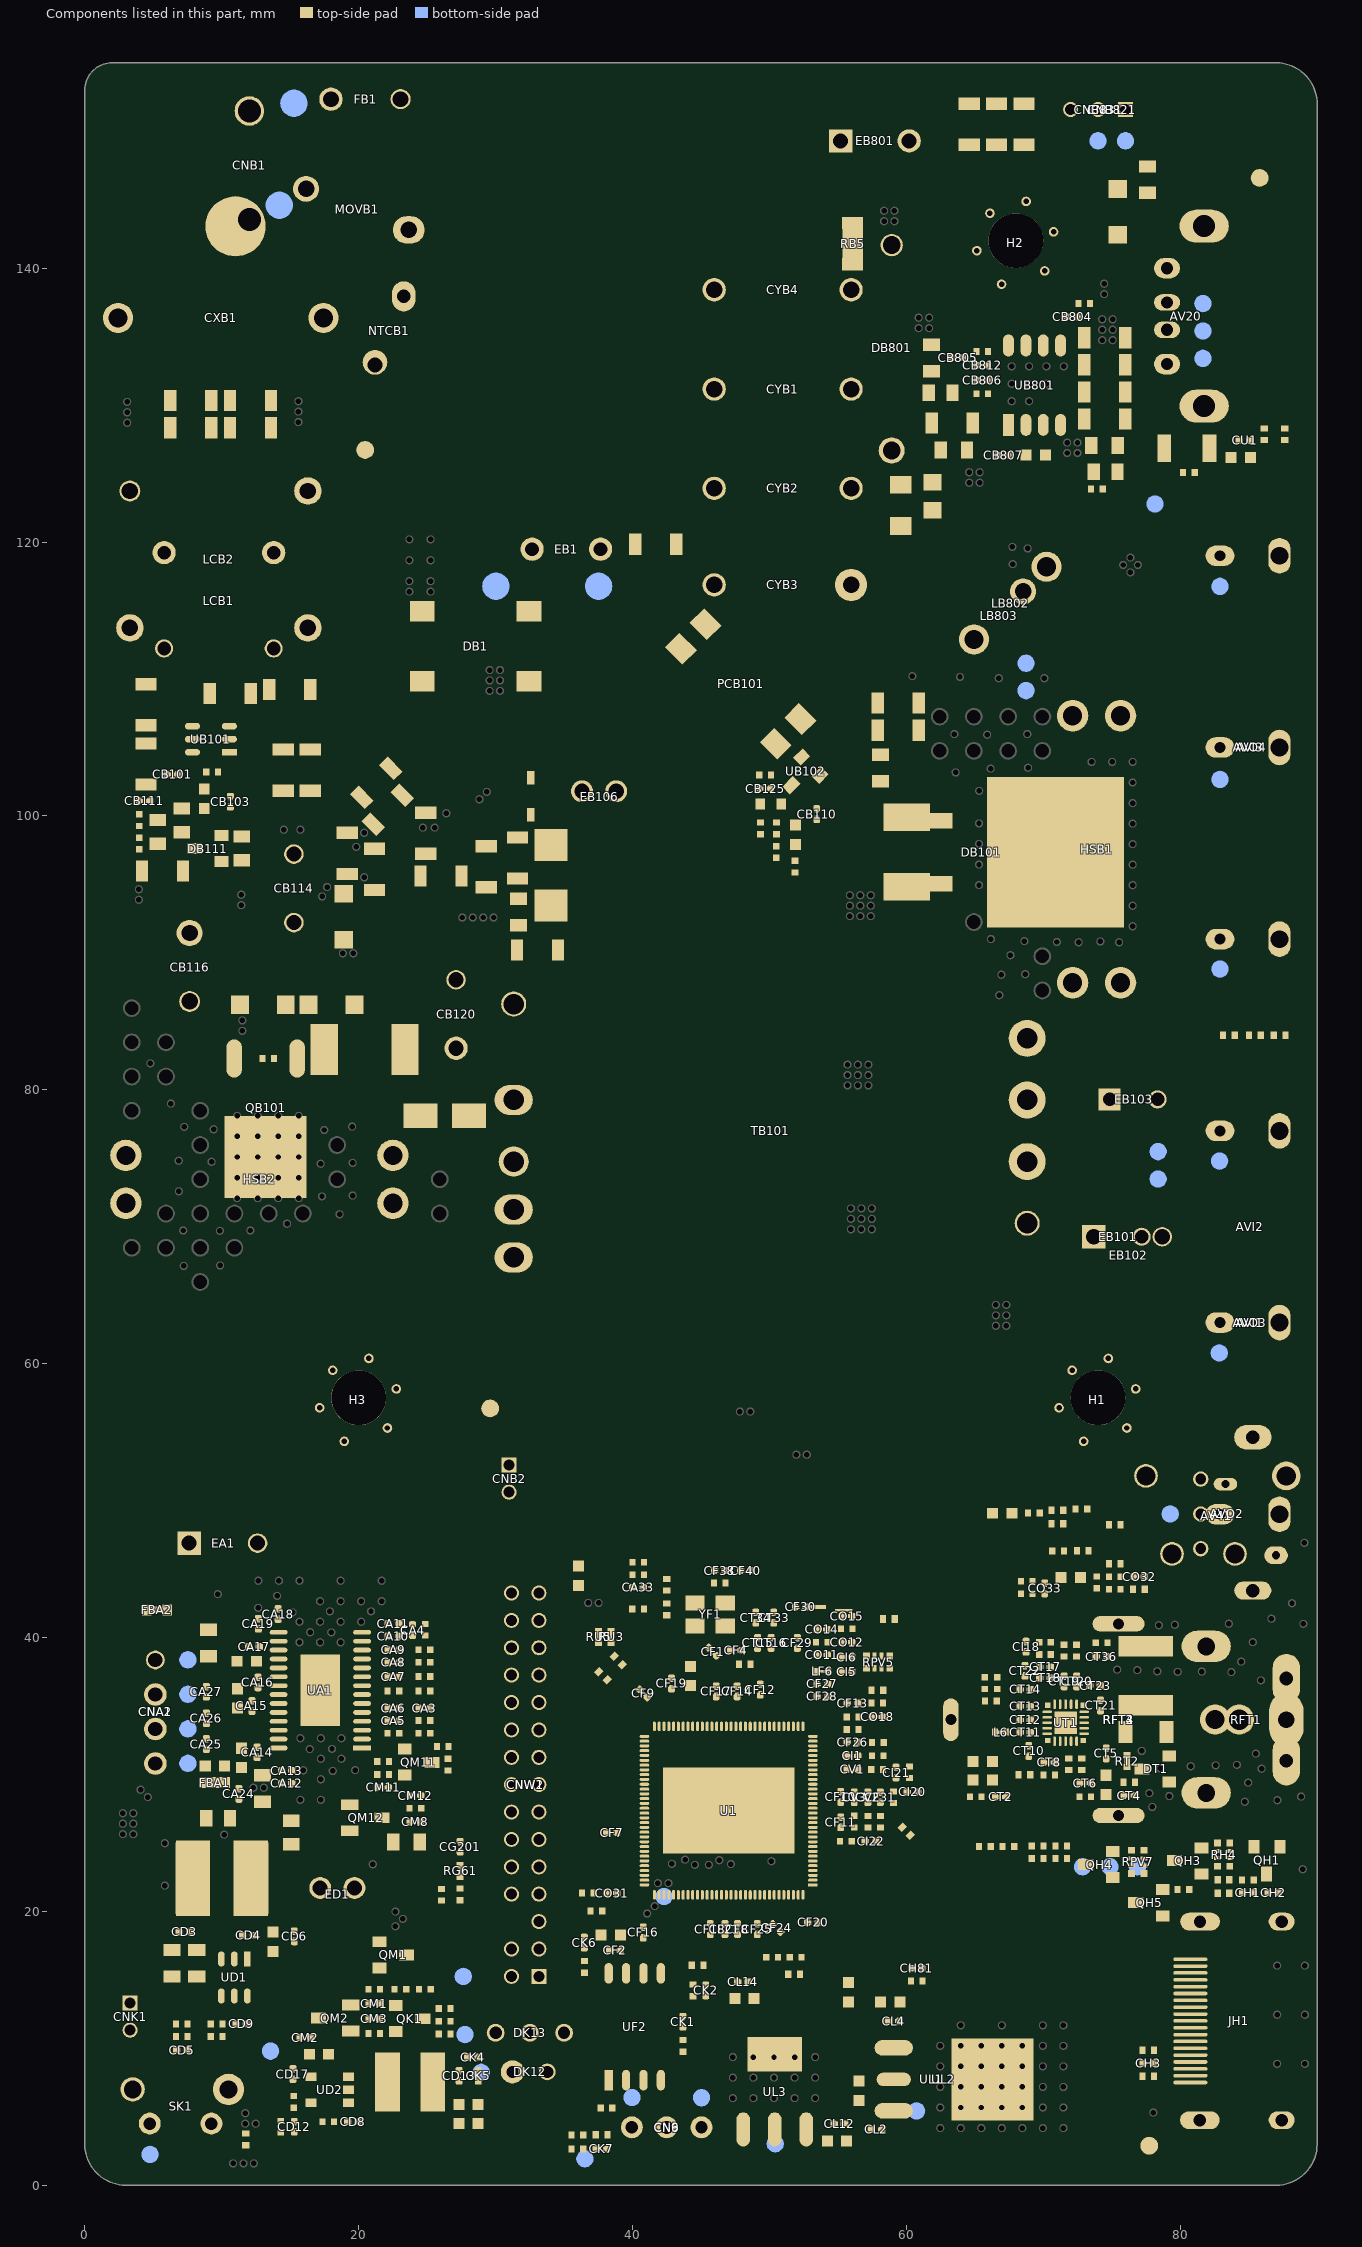
[diagram p0: the components of this part, seen from the top]
# Altium PCB MISC116569.PcbDoc (part 5 of 15)
Units mm, origin at the board's own origin, x right, y up, seen from the top; angles counter-clockwise.
Board outline 90 x 155 mm, 2 copper layers (TopLayer, BottomLayer), stack 1.571 mm thick; 527 components, 277 nets, 2450 pads, 649 vias.

## Footprints (in the part's own frame and the unit in brackets; to place one, negate y for a bottom-side part, rotate by r counter-clockwise, add the part's x,y. Pads: shape width x height; smd on the part's side, far side on the other; paste and mask are expansions set on the pad) (continued)
TO-252 [mm] "与TO-223兼容；15.12.29"
  oval 1.143x2.794 smd: 1(-2.3,-3.6) 3(2.3,-3.6)
  rect 6x6 smd paste-10: 2(0,3.6)
  rect 4x2.6 on Top Paste: 4(0,1.957)
  TopLayer pour cut-out: 2.3,-1.932 2.3,-5.055 -2.345,-5.055 -2.64,-4.996 -2.891,-4.829 -3.058,-4.579 -3.117,-4.284 -3.117,-4.284 -2.299,-4.284 -2.299,-2.699 -3.124,-2.699 -3.066,-2.406 -2.899,-2.157 -2.65,-1.99 -2.356,-1.932 -2.356,-1.932
  silkscreen extent -3.4,-1.34 3.4,7.01, body extent -3.4,-4.15 3.4,6.05, height 2.5
TO-252-GDS [mm] "SC08440  IRLR024N"
  rect 6x6 smd: D(0,0)
  oval 1.143x2.794 smd: G(-2.3,-7.2) S(2.3,-7.2)
  silkscreen extent -3.4,-5.64 3.4,3.4, body extent -3.4,-7.75 3.4,2.45, height 2.5
TP [mm] "TEST POINT   (不带paste  1.27mm 直径）"
  round 1.27 smd paste-1.27: 1(0,0)
TP-80 [mm] "TEST POINT;2mm"
  round 2 smd paste-1.27: 1(0,0)
TP-TDT [mm] "电源放电测试点，间隔7.5mm"
  round 2 smd paste-2: 1(-3.75,0) 2(3.75,0)
  silkscreen extent -5.75,-2 5.75,2
TP_BL [mm] "TEST POINT,专用背光测试点"
  round 1.27 smd paste-1.27: 1(0,0)
  silkscreen extent -6.4,-0.97 0.95,0.96
TSOT23-6 [mm] "MP65151DJ[MPS]/MP1470"
  rect 1.1x0.5 smd: 1(-1.35,0.95)
  oval 1.1x0.5 smd: 2(-1.35,0) 3(-1.35,-0.95) 4(1.35,-0.95) 5(1.35,0) 6(1.35,0.95)
  silkscreen extent -1.08,-1.5 0.85,2.8, body extent -0.85,-1.5 0.85,1.5, height 1
USB1-HD-2 [mm] "捷仕泰 ： U2504M-04-E1WD-C；170204加宽后壳丝印(18.03.12,更新信号脚孔径）"
  oval 2.7x3.9 on Top Overlay: 0(-6.57,10.257) 0(6.57,10.247)
  oval 1.7x2.1 on Top Overlay: 0(-3.5,12.957) 0(3.5,12.957)
  oval 1.5x1.9 hole 0.9 slot 1.4 at 90 deg: 1(-3.5,12.957) 4(3.5,12.957)
  oval 1.4x2.1 on Top Overlay: 1(-1,12.957) 2(1,12.957)
  oval 1.2x1.9 hole 0.9 slot 1.4 at 90 deg: 2(-1,12.957) 3(1,12.957)
  oval 2.4x3.6 / inner oval 2.4x3.6 / far side oval 2.8x4 hole 1.6 slot 2.3 at 90 deg: 5(6.57,10.247) 6(-6.57,10.247)
  TopLayer pour cut-out: 2.433,14.667 4.428,14.667 4.532,14.647 4.62,14.588 4.678,14.5 4.699,14.396 4.699,14.396 4.699,11.335 4.68,11.238 4.625,11.156 4.542,11.101 4.445,11.081 4.445,11.081 2.422,11.081 2.422,14.656
  KeepOutLayer pour cut-out: -3.49,14.696 -4.146,14.566 -4.703,14.194 -5.075,13.637 -5.206,12.98 -5.206,12.98 -5.206,12.94 -5.068,12.25 -4.677,11.665 -4.092,11.275 -3.402,11.137 -3.402,11.137 2.42,11.137 2.637,11.18 2.821,11.303 2.943,11.487 2.986,11.703 2.986,11.703 2.986,14.149 2.944,14.361 2.824,14.541 2.644,14.661 2.432,14.704 2.432,14.704 -3.482,14.704 -3.485,14.703 -3.487,14.701 -3.489,14.699 -3.49,14.696
  silkscreen extent -7.1,2.04 7.05,14.58, body extent -10,-87.25 10,14.14, height 8.2
VR(13*5)-V-7.5 [mm] "为勤,VARISTOR,17.01.04修改为椭圆孔;160105更新椭圆孔 //0424_2019在顶层加整块白油,"
  oval 2.311x2 / inner oval 2.8x2 / far side oval 2.8x2 hole 1.2 slot 2 at 0 deg: 1(3.75,-1.5)
  round 1.9 hole 1.2: 2(-3.75,1.5)
  round 2.1 on Top Overlay: 2(-3.75,1.5)
  oval 3x2.2 on Top Overlay: 2(3.75,-1.5)
  silkscreen extent -6.65,-2.5 6.44,2.5, body extent -6.5,-2.75 6.5,2.75, height 15.5
XTAL-S-3 [mm] "三星（SQ3D03200D2IBA）晶振"
  rect 1.4x1.1 smd: 1(-1.1,-0.85) 2(1.1,-0.85) 3(1.1,0.85) 4(-1.1,0.85)
  silkscreen extent -2.37,-1.91 1.65,1.3, body extent -1.65,-1.3 1.65,1.3, height 0.8

## Part data
5V CVBS_IN DM0 DP0 GND LOUT+ LOUT- PWM_REF ROUT+ ROUT- TP_12VA+ TP_12VA- TP_12VB+ TP_12VB- TP_L TP_LED+ TP_LED- TP_N UART_RX UART_TX Y_Pb_LOUT Y_Pr_ROUT Y_Y_AV_OUT YPBPR_L/AV_L YPBPR_R/AV_R: library part TEST
AV20: library part XXX.XXX.0002687, "USB jack,USB Jack,H,Single,flange,DIP,103411271,VAST-DLMI"
AV41: library part XXX.XXX.0002138, "Earphone jack,Earphone Jack,H,Φ3.5,CH7.0,Black,switch,Seal,DIP,PJ7724-F05L3BY-D,YUQIU-DLMI"
AVI1 AVO4: library part "RCA端子,RCA Jack,AV3,H,Yellow、White、Red,CH5.5,D14,Seal,DIP,RC075-F03L3BY-A,YUQIU-DLMI-AV", "CN-AV-D14-#-#"
AVI2: library part "RCA端子,RCA Jack,AV2,H,White、Red,CH5.5,D14,Seal,DIP,AV63-02S-0030,QS(MI手插物料)-DLMI-AUDIO", "CN-AUDIO-D14-#-#"
AVI3: library part "RCA端子,RCA Jack,AV3,H,Green、Blue、Red,CH5.5,D14,Seal,DIP,RC075-F03L3BY-B,YUQIU-DLMI-YPbPr", "CN-YPbPr-D14-#-#"
AVO2: library part GQ-03-08-DLMI, "CN-DLMI-optical fiber"
AVO3: library part "RCA端子,RCA Jack,AV3,H,Orange、White、Red,CH5.5,D14,Seal,DIP,RC075-F03L3BY-C,YUQIU-DLMI"
BA1 BA2 BA3 BA4: library part 004.004.0000104-D, "Multilayer inductor,HF Inductor,220nH,±5%,0603,SMD,SWI0603F-R22J,Tai-tech-D"
BB101: library part 004.004.0001046-D, "Ferrite bead,BEAD,50ohm,3.0×4.0,9A,SMD,TP,SMB-302540-K5B-L1,SOLDIER-D"
BB801: library part UPZ2012E601-2R0TF(600ohm-2000mA)
BB802: library part 004.004.0000340-D, "Ferrite bead,BEAD,600ohm±25%,0805,2000mA,SMD,TP,UPZ2012E601-2R0TF,Sunlord-D"
BOE: library part PCB_NAME
CA1 CA2 CD1 CD2 CM7: library part 004.003.0000386-D, "Ceramic capacitor,CAP MC,16V,10uF,±20%,X5R,0805,SMD,TP-D"
CA3 CA4: library part 004.003.0000549-D, "Ceramic capacitor,CAP MC,50V,3300pF,±10%,X7R,0402,SMD,TP-D"
CA5 CA6 CA10 CA11 CA14 CA15 CA16 CA17: library part 004.003.0000398-D, "Ceramic capacitor,CAP MC,16V,0.22uF,±20%,X5R,0402,SMD,TP-D"
CA7 CA9: library part 004.003.0000402-D, "Ceramic capacitor,CAP MC,16V,1uF,±20%,X5R,0402,SMD,TP-D"
CA8 CA12 CA18 CD3 CD4 CD6 CD8 CD9 CL2 CL12 CM1 CM2 CM8 CO32: library part 004.003.0000403-D, "Ceramic capacitor,CAP MC,16V,0.1uF,±20%,X5R,0402,SMD,TP-D"
CA13 CA19: library part 004.003.0000503-D, "Ceramic capacitor,CAP MC,50V,1000pF,±10%,X7R,0402,SMD,TP-D"
CA24 CA25 CA26 CA27: library part 004.003.0000534-D, "Ceramic capacitor,CAP MC,50V,2200pF,±10%,X7R,0402,SMD,TP-D"
CA31 CA32 CD7 CL13: library part 004.003.0000383-D, "Ceramic capacitor,CAP MC,6.3V,10uF,±20%,X5R,0603,SMD,TP-D"
CA33 CO12 CO15: library part 004.003.0000361-D, "Ceramic capacitor,CAP MC,6.3V,0.47uF,±10%,X5R,0402,SMD,TP-D"
CB101 CB111 CB807: library part 100pF-0402-NPO-±5%-50V-D
CB102 CB109: library part 0.1uF-0603-X7R-±10%-50V-D, "CAP"
CB103 CB806 CF29 CF30 CO11 CO14 CO18: library part 1000pF-0402-X7R-±10%-50V-D
CB110 CB125: library part 1000pF-0402-X7R-±10%-50V-D, "CAP"
CB113 CB808 CB809 CB810 CB811: library part 220PF-0805-NPO-±10%-200V-D, "CAP"
CB114: library part C242G472J20A201(编带/法拉)-DAI, "CAP"
CB116: library part 004.003.0001889-DHAI, "Ceramic capacitor,CAP CD,1KV,100pF,±5%,SL,OK,5.0mm,DIP,TP,TDK-DHAI"
CB118: library part 1000pF-0805-NPO-±10%-200V-D, "CAP"
CB120: library part 004.003.0001665, "Ceramic capacitor,CAP CD,1KV,4700pF,±20%,Y5U,K,5.0mm,DIP,TP,Walsin-DHAI"
CB801: library part 1uf-0603-X7R-±10%-25V-D
CB804: library part 4700pF-0402-X7R-±10%-50V-D
CB805: library part 0.1uF-0402-X7R-±10%-16V-D
CB812: library part 0.033uF-0402-X7R-±10%-16V-D
CD5: library part 004.003.0000570-D, "Ceramic capacitor,CAP MC,50V,56pF,±5%,NPO,0402,SMD,TP-D"
CD10 CD14 CD15 CD16 CF3 CF5 CF15 CL1 CL3 CL11 CT1 CT52 CU2: library part 10uF-0603-X5R-±20%-6.3V-D
CD12: library part 3300pF-0402-X7R-±10%-50V-D
CD13 CD17 CH1 CH2 CK4 CK5 CM11: library part 0.1uF-0402-X5R-±20%-16V-D
CF1 CF4: library part 004.003.0000527-D, "Ceramic capacitor,CAP MC,50V,18pF,±5%,NPO,0402,SMD,TP-D"
CF2 CF7 CF8 CF9 CF10 CF12 CF13 CF14 CF17 CF27 CG201 CI5 CI6 CK1 CT2 CT4 CT5 CT6 CT7 CT8 CT9 CT10 CT11 CT12 CT15 CT16 CT17 CT18 CT21 CT22 CT23: library part 0.1uF-0402-Y5V-+80%-20%-16V-D
CF11 CF16 CF18 CF19 CF20 CF21 CF25 CF28 CH81 CK7 CU1: library part 1uF-0402-X5R-±20%-6.3V-D
CF24: library part 004.003.0000100-D, "Ceramic capacitor,CAP MC,6.3V,2.2uF,±20%,X5R,0402,SMD,TP-D"
CF26 CF31 CI1 CV1 CV2 CV3: library part 0.047uF-0402-X7R-±10%-16V-D
CF38 CF40 CI18: library part 30pF-0402-NPO-±5%-50V-D
CH3: library part 004.003.0000530-D, "Ceramic capacitor,CAP MC,50V,22pF,±5%,NPO,0402,SMD,TP-D"
CI20 CI21 CI22 CK6: library part 10pF-0402-NPO-±5%-50V-D
CK2: library part 0.01uF-0402-X7R-±10%-50V-D
CL4 CL14: library part 004.003.0000382-D, "Ceramic capacitor,CAP MC,6.3V,1uF,±20%,X5R,0402,SMD,TP-D"
CM3 CM12: library part 0.022uF-0402-X7R-±10%-16V-D
CN6: library part 004.008.0000361-DHMI, "IR receiver,IR Receriver,2.5V~6V,38K,DIP,FDI-M6069560R538-WJGC25-D22,Fantasy-DHMI"
CN9: library part 004.008.0000501-DHMI, "IR receiver,IR Receriver,DIP,ARM-383AW1-Z-R-D10-22,ALL-BEST-DHMI"
CNA1: library part XXX.XXX.0000595-DHMI, "Connector socket,connect jack,4Pin,D2.50,D,L=2.8mm,DIP,CNJST-DHMI"
CNA2: library part XXX.XXX.0000676-DHMI, "Connector socket,connect jack,4Pin,D2.54,D,SNAP,L=3.0mm,DIP,BOOM-DHMI"
CNB1: library part "连接插座,connect jack,2Pin,D7.92,L,SNAP,Fool-proofing,nature,L=2.8mm,DIP,AMA-DLMI", "AC socket"
CNB2: library part XXX.XXX.0001753, "Connector socket,connect jack,2Pin,D2.0,D,L=2.8mm,DIP,AMA-DHMI"
CNB821: library part XXX.XXX.0000603-DHMI, "Connector socket,connect jack,2Pin,D2.0,D,L=3.4mm,DIP,BOOM-DHMI"
CNB831: library part XXX.XXX.0000643-DHMI, "Connector socket,connect jack,3Pin,D2.0,D,SNAP,L=2.8mm,DIP,CNJST-DHMI"
CNK1: library part 2PIN-2.0-D-H-G-B-DHMI, "Socket"
CNW1: library part 2×15PIN-2.0-D-H-M(脚长=2.6mm)(缺6PIN)-LK-DHMI, "CN-straight pin header"
CNW2: library part "连接插座,connect jack,2×15Pin/without pin6,D2.0,D,SNAP,Fool-proofing,Nature,L=2.6mm,DIP,CJ", "CN-with latch"
CO31 CT13 CT14 CT19 CT20 CT33 CT34 CT36: library part 33pF-0402-NPO-±5%-50V-D
CO33: library part 330pF-0402-NPO-±5%-50V-D
"Conformal Coating": library part 三防漆,25kg/Can,Peters
CT3: library part 1000pF-1206-X7R-±20%-2000V-D
CXB1: library part "X电容,CAP X2,MP,275VAC,0.47uF,±10%,S,15mm-Mini,PC,DIP,BM-DHMI", "CAP"
CYB1 CYB2 CYB3 CYB4: library part "Y电容,CAP Y1,CD,470pF,400VAC,±20%,KS,10mm,Y5U,DIP,Walsin-DHMI", "Y1 capacitor"
D101 D102 DA31 DA32 DA33 DI10 DI11 DK1 DK3 DV3 DV4 DV5 DV7 DV8 DV9: library part AVLC18S02003-D
DAS1: library part DOLBY_AS2
DB1: library part 004.005.0000860-D, "Bridge rectifier,DIO BRD,3A,800V,YBS,SMD,YBS3010A,YJ-D"
DB101: library part MBRB10150CT(GOOD-ARK)-D, "Diode"
DB104: library part M7(GOOD-ARK)-D
DB106 DB109 DB110 DB804: library part "整流二极管,DIO FRD S,1.2A,800V,eSGA,SMD,R12K,GOOD-ARK-D"
DB111: library part LBAV70LT1G(LRC)-D, "Diode"
DB121: library part BAV21WS-D, "Diode"
DB801: library part SR210(编带/台半)-DLAI, "Diode"
DH1 DH2 DH3 DH81: library part 004.005.0000315-D, "TVS diode,DIO ESD,2.5pF,200V,0402,SMD,SFI0402-240E-2R5PP-LF,SFI-D"
DI1 DI2 DI3: library part AIES12U020R2-D
DK12: library part "发光二极管,Single LED,RED,25mA,28mcd,638nm,1.9V,φ3.85×5.4mm,DIP,HL-DLMI"
DK13: library part WEJ3290C-R3H8-BC(红、绿)-高亮-DLMI
DT1: library part BAV99-BR-D
DU1 DU2 DU3 DU4: library part 004.005.0000203-D, "TVS diode,DIO ESD,0.2pF,25V,0402,SMD,AIES12U020R2,AMOTECH-D"
EA1: library part 004.003.0000601-DHAI, "Aluminum electrolytic capacitor,CAP AL,16V,470uF,±20%,RK,P,5.0mm,10×12,DIP,TP,XL-DHAI"
EB1: library part 47uF-400V-±20%-13×30-105℃-KY-折脚(H=11mm)(Capxon)-DLMI, "Electrolytic"
EB101 EB103: library part 270uF-16V-±20%-8×11.5-105℃-PS-短脚-F=3.5(Capxon), "Solid-state"
EB102: library part 470uF-25V-±20%-10×12.5-105℃-GF-编带-F=5.0(CapXon)-DHAI, "Electrolytic"
EB106: library part 10uF-50V-±20%-5×11-105℃-GH-编带-F=2.5(CapXon)-DHAI, "Electrolytic"
EB801: library part 47uF-100V-±20%-10×12-105℃-EV-编带-F=5.0(Elite)-DHAI, "Electrolytic"
ED1: library part 470uF-10V-±20%-6.3×11-105℃-黑底白字-编带-F=2.5-XF-DHAI, "Electrolytic"
EVA1 EVA2 EVA3 EVA4: library part 7×7×3mm-C-4305防火泡棉-黑色-DLMI, "EVA"
FB1: library part 004.026.0000010-DHMI, "Slow-blow fuse,FUSE T,P,3.15A,250VAC,8.5×4.0×8mm,DIP,TP,Walter-DHMI"
FBA1 FBA2: library part 0ohm-0603-PCB-D, "0ohm-0603-PCB-D"
FT2 LT1 LT3 LT4: library part SDCL1005CR27JTDF(顺络)-D
FU1: library part 004.026.0000039-D, "Resettable fuse,FUSE PTC,1.1A,6V,1206,SMD,TP,TLC-D"
GD1 GD2 GD3: library part 7.00×8.35mm-尼龙-白色-WQM-DHMI, "Mylar stud"
GDT1: library part 004.005.0000675, "Gas discharge tube,GDT,700V,2000A,TP,4.5*3.2mm,SMD,4532-091-LF,Brightking-D"
GL1 GL5 GL6 GL7 GL8: library part 005.002.0000011, "Silicone,0.2g,general purpose,60,White,SLD-8854W,XY-DHMI"
GL3 GL4: library part 005.002.0000011-D-5*3mm, "Silicone,0.5g,general purpose,60,White,SLD-8854W,XY-D"
H1 H2 H3: library part "Location hole-D"
HS1: library part 004.040.0008928-D, "Heat sink,15.0×15.0×5.0mm,AL1060H-24,Black,high-emissivity paint spray,stamped with bends,no rivet pins,YT-D"
HSB1 HSB2: library part 004.040.0006600-DHMI, "Heat sink,17.5×14.5×0.5mm,copper sheet,matte tin plated,natural color,four pins,WT-DHMI"
JH1: library part XXX.XXX.0001122-D, "HDMI jack,HDMI Jack,H,SMD,161031041(hull-SPCC ),VAST-D"
L3: library part FCM1005KF-121T06(120ohm-500mA)-D
L6 LF6 RG61 RT2 RU3 RU5: library part 0ohm-0402-PCB-D, "0ohm-0402-PCB-D"
LB802: library part SYDR1212-L003-HM-DHMI, "I-core inductor"
LB803: library part 差模电感,Inductor,DR12×14,68uH,0.45,20Ts,H13.5MAX,SYDR1214-L068uA,DIP,Soldier-DHMI, "I-core inductor"
LCB1: library part SYUU9.8-L002-JM-DLMI, "Common mode"
LCB2: library part SYUU10.5-L002-JM-DHMI, "Common mode"
LD1: library part 004.004.0000017-D, "Power inductor,Power Inductor,4.7uH,±20%,2.8A,0.35×1P,DR5.8×4.5,SMD,SCD54TL-4R7M,Soldier-D"
LD2: library part SLN43T-6R8M-D
LD3: library part 004.004.0000016-D, "Power inductor,Power Inductor,4.7uH,±20%,3.3A,DR6.0×4.5,SMD,SWPA6045S4R7MT,Sunlord-D"
LT2: library part MGLB1608M121T2R0-LF(120ohm-2000mA)-D
M1 M2 M3 M4: library part MARK-D
ML1: library part MALAY
MOVB1: library part TVR10561KSW(为勤)-DHMI, "Varistor"
NTCB1: library part SCK102R55AMBY502(短脚/为勤)-DHMI, "Thermistor"
PCB101: library part LTV-817S-TA-B(光宝)-DMI, "Optocoupler"
QB101: library part 场效应管,NMOS,5.2,650V,1.02ohm@ID=2.6A@VGS=10V,DPAK,TK5P65W,TOSHIBA-D, "N Channel Single MOSFET"
QH1 QM1: library part 004.006.0000007-D, "General-purpose transistor,Dynatron,NPN,0.2A,40V,60-300,SOT-23,KMBT3904,KEXIN-D"
QH3 QH4 QH5 QK1 QM11: library part LMBT3904LT1G-D-NPN, "Q-NPN-#-#-#"
QM2: library part 004.007.0000286-D, "MOSFET,PMOS,-4.7A,-20V,70mohm@ID=-4.7A@VGS=-4.5V,SOT23-LC,LPB3443LT1G,LRC-D"
QM12: library part WPM3407C-3/TR-D
R5V R12V: library part 0ohm-0805-±5%-1/8W-D
RA1 RA2 RM3: library part 004.002.0000689-D, "Thick-film resistor,RES,1/16W,4.7Kohm,±5%,0402,SMD-D"
RA3 RA14: library part 004.002.0000572-D, "Thick-film resistor,RES,1/16W,1Kohm,±5%,0402,SMD-D"
RA4 RA5: library part GND
RA8 RD1 RD7 RM4: library part 004.002.0000579-D, "Thick-film resistor,RES,1/16W,100Kohm,±5%,0402,SMD-D"
RA9: library part 004.002.0000691-D, "Thick-film resistor,RES,1/16W,47Kohm,±5%,0402,SMD-D"
RA10: library part 004.002.0000575-D, "Thick-film resistor,RES,1/16W,10Kohm,±1%,0402,SMD-D"
RA11: library part 004.002.0000602-D, "Thick-film resistor,RES,1/16W,15Kohm,±1%,0402,SMD-D"
RA25 RH83 RH88 RH89 RO22: library part 004.002.0000568-D, "Thick-film resistor,RES,1/16W,100ohm,±5%,0402,SMD-D"
RA31 RA32 RF25 RH3 RK3 RK10: library part 1Kohm-0402-±5%-1/16W-D
RA33 RA34 RO21: library part 004.002.0000609-D, "Thick-film resistor,RES,1/16W,180ohm,±5%,0402,SMD-D"
RA35 RM14: library part 47Kohm-0402-±5%-1/16W-D
RA36 RB804 RH59 RK15 RM12: library part 10Kohm-0402-±5%-1/16W-D
RB1 RB2 RB3 RB4: library part 1M2ohm-1206-±5%-1/4W-D, "RES"
RB5: library part 0ohm-1206-PCB-D, "0ohm-1206-PCB-D"
RB101 RB102 RB161 RB162 RB163: library part 330Kohm-1206-±5%-1/4W-D, "RES"
RB103: library part 6K8ohm-0402-±1%-1/16W-D
RB104: library part 47Kohm-0402-±1%-1/16W-D
RB105: library part 510ohm-0402-±1%-1/16W-D
RB106 RB121: library part 68ohm-0805-±5%-1/8W-D
RB107: library part 20ohm-0805-±5%-1/8W-D, "RES"
RB109 RB133 RB803: library part 10Kohm-0402-±1%-1/16W-D
RB114: library part 4R7ohm-1206-±1%-1/4W-D, "RES"
RB116 RB117 RB118 RB119 RB810 RB812: library part 10ohm-1206-±5%-1/4W-D, "RES"
RB123 RB124: library part 47ohm-1206-±5%-1/4W-D, "RES"
RB125 RB126 RB127 RB128: library part 100Kohm-1206-±5%-1/4W-D, "RES"
RB130: library part 20ohm-1206-±5%-1/4W-D
RB131: library part 1Kohm-0603-±1%-1/10W-D
RB132: library part 1Kohm-0402-±1%-1/16W-D
RB134: library part 4K7ohm-0402-±1%-1/16W-D, "RES"
RB135: library part 18Kohm-0402-±1%-1/16W-D, "RES"
RB141 RB142: library part 2Mohm-1206-±5%-1/4W-D, "RES"
RB148: library part 厚膜电阻,RES,1W,0.24ohm,±1%,2512,SMD
RB158: library part 3Kohm-0402-±1%-1/16W-D
RB801 RB805 RK18 RK19: library part 100ohm-0402-±5%-1/16W-D
RB814: library part 390Kohm-0805-±1%-1/8W-D, "RES"
RB816: library part 33ohm-0805-±5%-1/8W-D
RB818: library part 0R2ohm-1206-±1%-1/4W-D
RB819 RB820: library part 0R1ohm-1206-±1%-1/4W-D
RB837: library part 1R6ohm-1206-±1%-1/4W-D, "RES"
RB838 RB839: library part 2R2ohm-1206-±1%-1/4W-D, "RES"
RD3: library part 004.002.0000104-D, "Thick-film resistor,RES,1/16W,33Kohm,±1%,0402,SMD-D"
RD5: library part 004.002.0000717-D, "Thick-film resistor,RES,1/16W,6.04Kohm,±1%,0402,SMD-D"
RD6: library part 004.002.0000806-D, "Thick-film resistor,RES,1/16W,60.4Kohm,±1%,0402,SMD-D"
RD8: library part 004.002.0000593-D, "Thick-film resistor,RES,1/16W,13Kohm,±1%,0402,SMD-D"
RD9: library part 004.002.0000588-D, "Thick-film resistor,RES,1/16W,12Kohm,±1%,0402,SMD-D"
RF3 RF8 RF9 RF13 RF29 RF43 RF44 RK12 RM11 RM13 RM15: library part 4K7ohm-0402-±5%-1/16W-D
RF12 RF16: library part 68ohm-0402-±5%-1/16W-D
RFT1: library part "RF头,RF JACK,H,IEC,T14.5,CH6.3,12.4×13.2×7.7mm,DIP,LHD-020组件,LHD-DLMI", "T-IEC-6.3mm-#-#"
RFT2: library part "RF屏蔽罩,RF SHLED,Single,H,IEC,T14.5,CH6.3,whole,14.5×25×9,DIP,122010461,VAST-DLMI", "T-IEC-14.5×25×9, head length 14.5-#-#"
RFT3: library part T-25×14.5×9-IEC14.5-LHD(3只脚)-DLMI, "T-IEC-14.5×25×9, head length 14.5-one-piece 3 pins-#"
RFT4: library part "RF屏蔽罩,RF SHLED,Single,H,F,T14.5,CH6.3,whole,25.0×14.5×10.0mm,DIP,T-14.5×25×10-F14.5-LHD (一体),LHD-DLMI", "T-F-14.5×25×10, head length 14.5-#-#"
RH4 RPV5 RPV7: library part 4*100ohm-0402-±5%-1/16W-D
RH5 RH6 RI3 RO4 RV2 RV4 RV10: library part 33ohm-0402-±5%-1/16W-D
RH81: library part 22Kohm-0402-±5%-1/16W-D
RH82 RK13: library part 33Kohm-0402-±5%-1/16W-D
RI15 RI16 RO17 RU4: library part 004.002.0000558-D, "Thick-film resistor,RES,1/16W,0ohm,±5%,0402,SMD-D"
RI18 RO18 RV1 RV3 RV5: library part 75ohm-0402-±5%-1/16W-D
RK4: library part 4K7ohm-0402-±1%-1/16W-D
RK14 RO12 RO15: library part 510ohm-0402-±5%-1/16W-D
RM1 RM2: library part 004.002.0000577-D, "Thick-film resistor,RES,1/16W,10Kohm,±5%,0402,SMD-D"
RO2 RT1: library part 0ohm-0402-±5%-1/16W-D
RT5 RT10 RT12 RT13 RT14 RT15: library part 220ohm-0402-±5%-1/16W-D
SFQ1 SFQ2 SFQ3 SFQ4: library part SFQ-D, "NC/Conformal coating,25kg/Can,Peters-D"
SK1: library part "轻触开关,Tact Switch,160±50gf,7.0×10.3×7.0mm,DIP,KFC-A06-E-4-7.5/4(R),YK-DLMI"
TB101: library part 004.004.0002645-DLMI, "变压器,Transformer,EQ2414,300uH,0.2×1P,26Ts,H14.5MAX,SYEQ2414Z-T012064B(BLACK),DIP,SQ-DLMI"
TP-TDT: library part TEST, "TEST"
U1: library part 004.016.0001146-D, "TV main chip,IC Main Chip,TSUMV53RWUT-Z1,32bit,Single-Core,QFN128,SMD,Mstar-D"
UA1: library part 004.012.0000275-D, "Audio amplifier,IC Audio AMP,Class D,2X8W@12V@8ohm,E-TSSOP-28L,SMD,AD52050B-26QG28NRR,ESMT-D"
UB101: library part "PWM控制器,IC PWM Controller,65KHZ,SOT23-6,SMD,OB2273C,ON-Bright-D", "IC"
UB102: library part AZ431AN-ATRE1(BCD)-D, "SMD 431"
UB801: library part "PWM控制器,IC PWM Controller,120KHz,SOP-8,SMD,OB3353LCPA,ON-Bright-D", "IC"
UD1: library part 004.010.0001184-D, "DC-DC converter,IC DC-DC,Syn,2A,18V,600KHz,SOT23-6,SMD,TMI3252T,TOLL-D"
UD2: library part "DC-DCоƬ,IC DCDC,Syn,1.2A,7.0V,1.5MHz,SOT23-5,SMD,LC2127CB5TR,Leadchip-D"
UF2: library part "SPI FLASH оƬ,IC SPI FLASH,32Mb,SOIC8,SMD,GD25Q32CSIG,GigaDevice-D"
UL1 UL3: library part 004.010.0000061-D, "LDO regulator,IC LDO,1A,1.8V,12V,SOT-223,SMD,LC1117CLTR18,Leadchip-D"
UL2: library part 004.010.0000064-D, "LDO regulator,IC LDO,1A,3.3V,12V,TO-252,SMD,LC1117COTR33,Leadchip-D"
UT1: library part 004.014.0000255-D, "Silicon tuner chip,IC Si Tuner,QFN-24,SMD,ATBM253,AltoBeam-D"
YF1: library part 16.000MHz±20PPM-10PF-SMD3225-D
用于U1上: library part Φ12mm×12mm-黑色-125度(UL认证)-D